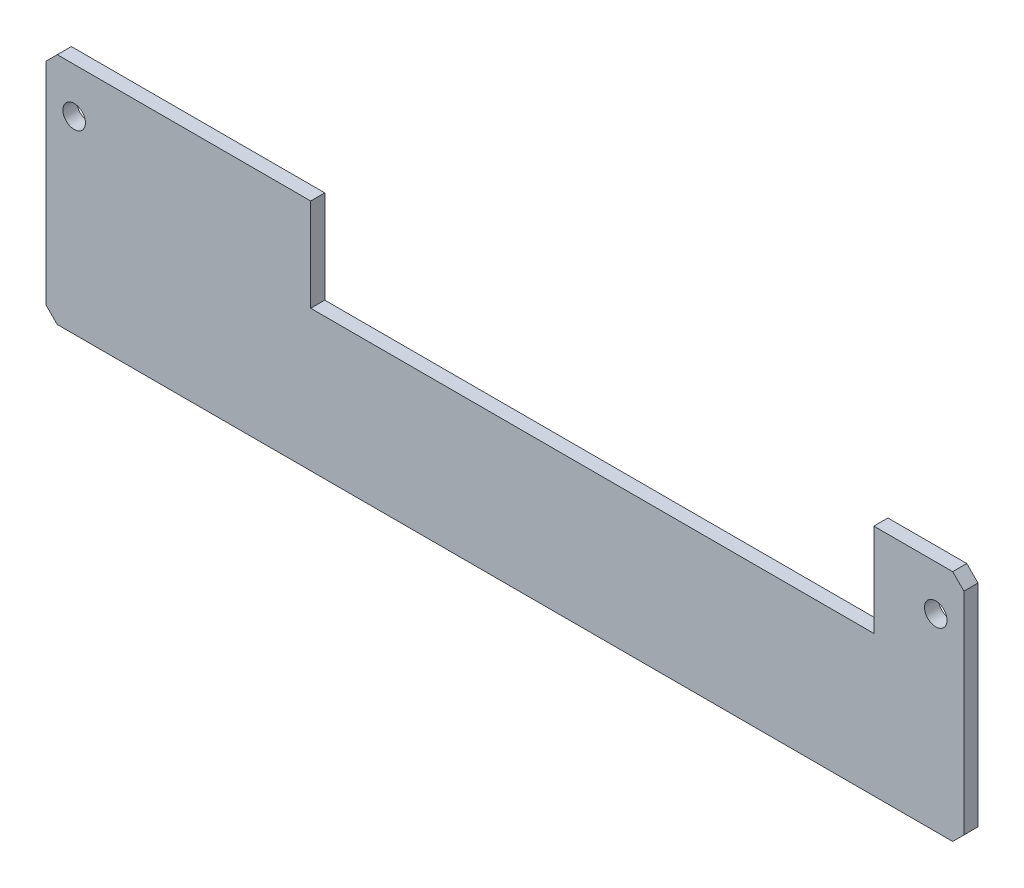
SolidWorks part; units mm, degrees
ref_plane "Front Plane" through (0, 0, 0) normal (0, 0, 1) x (1, 0, 0)
ref_plane "Top Plane" through (0, 0, 0) normal (0, 1, 0) x (1, 0, 0)
ref_plane "Right Plane" through (0, 0, 0) normal (1, 0, 0) x (0, 0, -1)
sketch "Sketch1" plane through (0, 0, 0) normal (0, 0, 1) x (1, 0, 0)
  line L1 (815, 207.5) -> (-815, 207.5)
  line L2 (815, 207.5) -> (815, -207.5)
  line L3 (815, -207.5) -> (-815, -207.5)
  line L4 (-815, 207.5) -> (-815, -207.5)
  line L5 (815, 207.5) -> (-815, -207.5) construction
  line L6 (815, -207.5) -> (-815, 207.5) construction
  point P0 (0, 0)
  dimension "D1" = 1630
  dimension "D2" = 415
extrude "Boss-Extrude1" add sketch "Sketch1" along normal blind 25
chamfer "Chamfer1" distance 20 angle 45 4 edges at (-815, -207.5, 12.5) (815, -207.5, 12.5) (815, 207.5, 12.5) (-815, 207.5, 12.5)
sketch "Sketch2" plane through (0, 0, 25) normal (0, 0, 1) x (1, 0, 0)
  line L5 (-815, 187.5) -> (-815, -187.5) construction
  line L6 (795, 207.5) -> (-795, 207.5) construction
  line L7 (815, -187.5) -> (815, 187.5) construction
  line L8 (-345, 42.5) -> (655, 42.5)
  line L9 (-345, 42.5) -> (-345, 242.5)
  line L17 (-345, 242.5) -> (655, 242.5)
  line L18 (655, 42.5) -> (655, 242.5)
  circle A0 centre (-765, 127.5) radius 20
  circle A1 centre (765, 127.5) radius 20
  dimension "D8" = 40
  dimension "D4" = 50
  dimension "D5" = 80
  dimension "D6" = 50
  dimension "D7" = 80
extrude "Cut-Extrude1" cut sketch "Sketch2" against normal through all both and the other way through all
